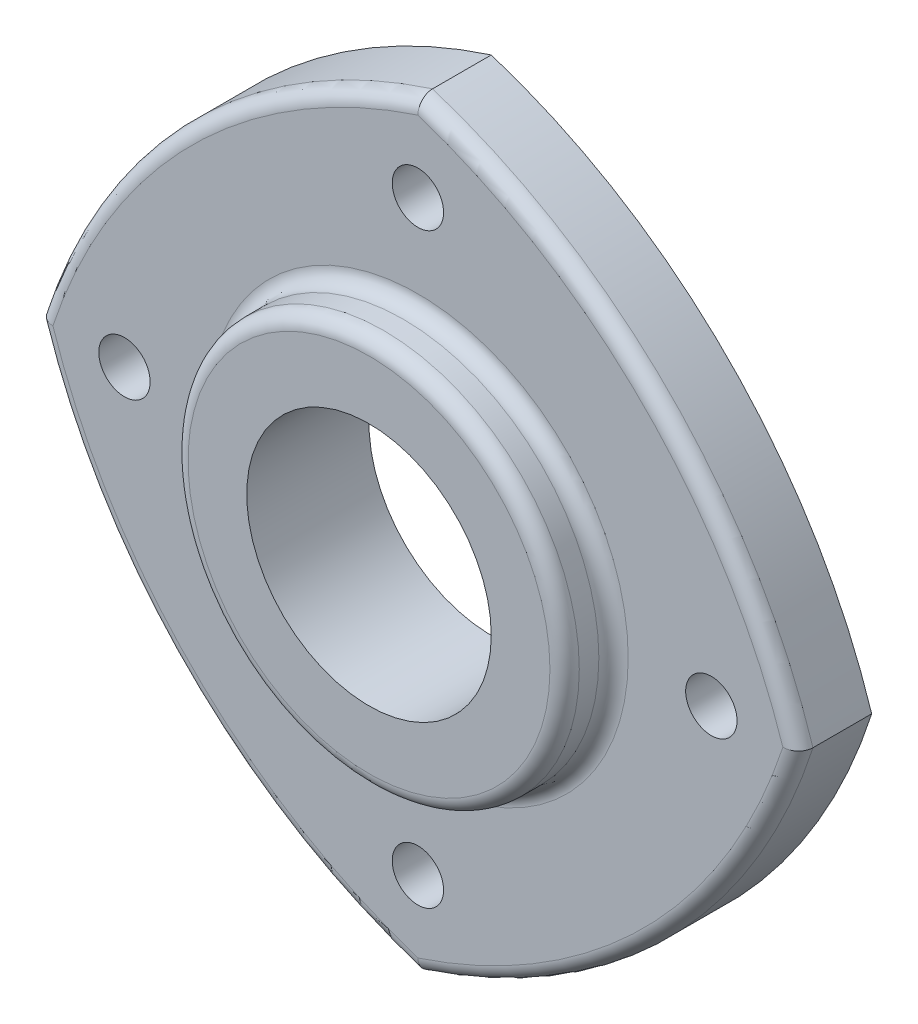
SolidWorks part; units mm, degrees
material "普通碳钢"
ref_plane "前视基准面" through (0, 0, 0) normal (0, 0, 1) x (1, 0, 0)
ref_plane "上视基准面" through (0, 0, 0) normal (0, 1, 0) x (1, 0, 0)
ref_plane "右视基准面" through (0, 0, 0) normal (1, 0, 0) x (0, 0, -1)
sketch "草图1" plane through (0, 0, 0) normal (0, 0, 1) x (1, 0, 0)
  line L0 (0, 77.7817) -> (77.7817, 0) construction
  line L1 (0, 77.7817) -> (-77.7817, 0) construction
  line L2 (77.7817, 0) -> (0, -77.7817) construction
  line L3 (-77.7817, 0) -> (0, -77.7817) construction
  line L4 (0, 77.7817) -> (0, -77.7817) construction
  line L5 (77.7817, 0) -> (-77.7817, 0) construction
  line L6 (0, 0) -> (0, 87.4399) construction
  line L7 (0, 0) -> (112.6345, 0) construction
  circle A0 centre (0, 60) radius 5.25
  circle A1 centre (60, 0) radius 5.25
  circle A2 centre (0, -60) radius 5.25
  circle A3 centre (-60, 0) radius 5.25
  arc A4 (0, 77.7817) -> (77.7817, 0) centre (-36.5246, -36.5246) cw
  arc A5 (-77.7817, 0) -> (0, 77.7817) centre (36.5246, -36.5246) cw
  arc A6 (-77.7817, 0) -> (0, -77.7817) centre (36.5246, 36.5246) ccw
  arc A7 (0, -77.7817) -> (77.7817, 0) centre (-36.5246, 36.5246) ccw
  point P1 (0, 0)
  point P20 (0, 0)
  dimension "D4" = 10.5
  dimension "D7" = 120
  dimension "D8" = 120
  dimension "D9" = 120
  dimension "D10" = 120
  dimension "D1" = 110
  dimension "D2" = 110
  dimension "D3" = 45
  dimension "D5" = 60
  dimension "D6" = 4
extrude "凸台-拉伸1" add sketch "草图1" along normal blind 15
sketch "草图2" plane through (0, 0, 15) normal (0, 0, 1) x (1, 0, 0)
  circle A0 centre (0, 0) radius 40
  dimension "D1" = 80
extrude "凸台-拉伸2" add sketch "草图2" along normal blind 10
sketch "草图3" plane through (0, 0, 25) normal (0, 0, 1) x (1, 0, 0)
  circle A0 centre (0, 0) radius 25
  dimension "D1" = 50
extrude "切除-拉伸1" cut sketch "草图3" against normal through all
fillet "圆角1" radius 3 6 edges at (-48.3282, 48.3282, 15) (-48.3282, -48.3282, 15) (48.3282, -48.3282, 15) (48.3282, 48.3282, 15) (40, 0, 25) (-40, 0, 15)
